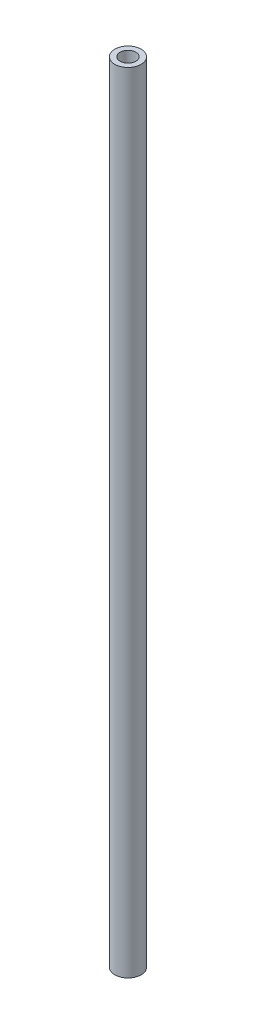
SolidWorks part; units mm, degrees
material "6061 合金"
ref_plane "前视基准面" through (0, 0, 0) normal (0, 0, 1) x (1, 0, 0)
ref_plane "上视基准面" through (0, 0, 0) normal (0, 1, 0) x (1, 0, 0)
ref_plane "右视基准面" through (0, 0, 0) normal (1, 0, 0) x (0, 0, -1)
other "Configuration Table"
sketch "草图1" plane through (0, 0, 0) normal (0, 1, 0) x (1, 0, 0)
  circle A0 centre (0, 0) radius 1.5
  circle A1 centre (0, 0) radius 2.5
  dimension "D1" = 3
  dimension "D2" = 5
extrude "凸台-拉伸1" add sketch "草图1" along normal blind 150
